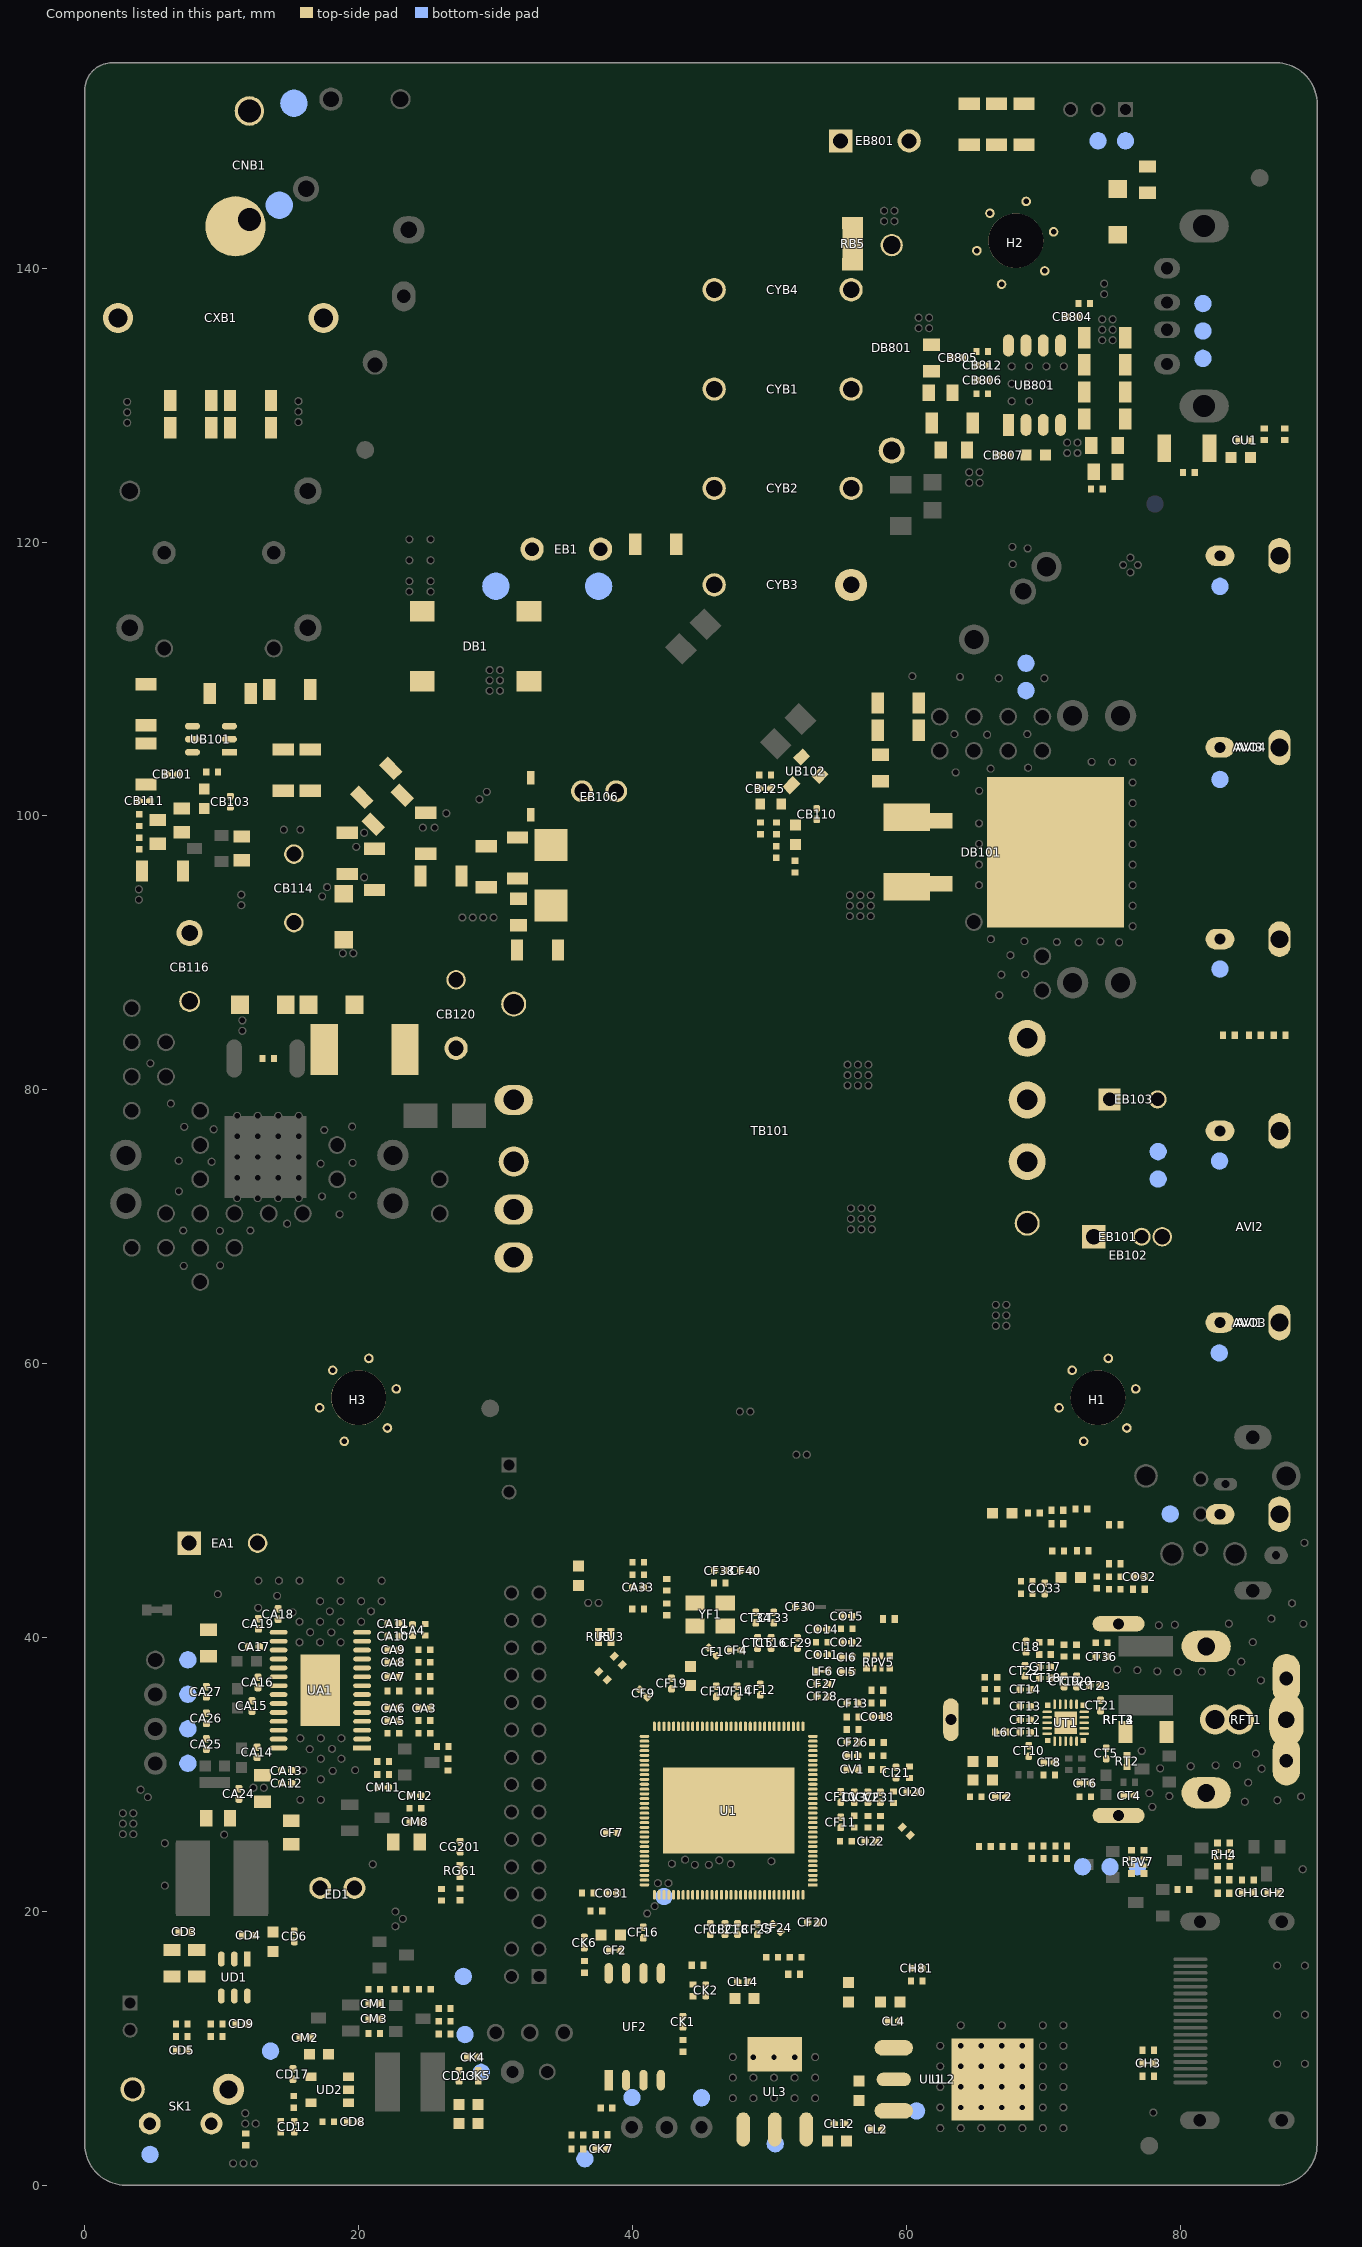
[diagram p0: the components of this part, seen from the top]
# Altium PCB MISC116569.PcbDoc (part 3 of 15)
Units mm, origin at the board's own origin, x right, y up, seen from the top; angles counter-clockwise.
Board outline 90 x 155 mm, 2 copper layers (TopLayer, BottomLayer), stack 1.571 mm thick; 527 components, 277 nets, 2450 pads, 649 vias.

## Components (designator, comment, footprint, x,y, rotation, side; value= is the part's Value field where it differs from the comment) (continued)
RA14 "1Kohm-0402-±1%-1/16W" R0402 24.862,40.57 r90 top
RA25 "10ohm-0402-±1%-1/16W" R0402 24.804,37.154 r0 top
RA31 "NC/1Kohm-0402-±1%-1/16W" R0402 75.217,44.44 r180 top
RA32 "NC/1Kohm-0402-±1%-1/16W" R0402 72.79,49.378 r180 top
RA33 "NC/Thick-film resistor,RES,1/16W,180ohm,±1%,0402,SMD" R0402 69.318,49.088 r0 top
RA34 "NC/Thick-film resistor,RES,1/16W,180ohm,±1%,0402,SMD" R0402 73.901,44.025 r90 top
RA35 "NC/47Kohm-0402-±1%-1/16W" R0402 40.419,45.494 r180 top
RA36 "NC/10Kohm-0402-±1%-1/16W" R0402 40.413,44.579 r0 top
RB1 "1M2ohm-1206-±5%-1/4W" R1206 12.103,130.341 r180 top
RB2 "1M2ohm-1206-±5%-1/4W" R1206 12.103,128.347 r180 top
RB3 "1M2ohm-1206-±5%-1/4W" R1206 7.73,128.351 r180 top
RB4 "1M2ohm-1206-±5%-1/4W" R1206 7.73,130.345 r180 top
RB5 "NC/Thick-film resistor,RES,1/4W,0ohm,±5%,1206,SMD" R1206SC 56.07,141.798 r90 top
RB101 "Thick-film resistor,RES,1/4W,330Kohm,±1%,1206,SMD" R1206 14.96,109.24 r180 top
RB102 "Thick-film resistor,RES,1/4W,330Kohm,±1%,1206,SMD" R1206 10.631,108.95 r180 top
RB103 "6K8ohm-0402-±1%-1/16W" R0402 3.975,99.695 r270 top
RB104 "47Kohm-0402-±1%-1/16W" R0402 9.296,103.2 r0 top
RB105 "510ohm-0402-±1%-1/16W" R0402 3.975,97.987 r270 top
RB106 "68ohm-0805-±5%-1/8W" R0805 11.455,97.638 r270 top
RB107 "20ohm-0805-±5%-1/8W" R0805 7.087,99.682 r270 top
RB109 "10Kohm-0402-±1%-1/16W" R0402 13.398,82.283 r180 top
RB114 "4R7ohm-1206-±1%-1/4W" R1206 33.06,90.208 r0 top
RB116 "NC/10ohm-1206-±5%-1/4W" R1206 31.598,96.926 r270 top
RB117 "Thick-film resistor,RES,1/4W,10ohm,±1%,1206,SMD" R1206 16.472,103.347 r90 top
RB118 "Thick-film resistor,RES,1/4W,10ohm,±1%,1206,SMD" R1206 14.488,103.347 r90 top
RB119 "Thick-film resistor,RES,1/4W,10ohm,±1%,1206,SMD" R1206 5.677,95.974 r0 top
RB121 "NC/Thick-film resistor,RES,1/8W,27Kohm,±1%,0805,SMD" R0805 5.334,98.842 r90 top
RB123 "47ohm-1206-±5%-1/4W" R1206 59.413,106.265 r0 top
RB124 "47ohm-1206-±5%-1/4W" R1206 59.413,108.246 r0 top
RB125 "Thick-film resistor,RES,1/4W,100Kohm,±1%,1206-Auto,SMD" R1206 19.168,97.262 r90 top
RB126 "Thick-film resistor,RES,1/4W,100Kohm,±1%,1206-Auto,SMD" R1206 21.285,102.413 r45 top
RB127 "Thick-film resistor,RES,1/4W,100Kohm,±1%,1206-Auto,SMD" R1206 21.161,96.094 r90 top
RB128 "Thick-film resistor,RES,1/4W,100Kohm,±1%,1206-Auto,SMD" R1206 22.123,100.457 r45 top
RB130 "Thick-film resistor,RES,1/4W,20ohm,±1%,1206,SMD" R1206 41.689,119.842 r0 top
RB131 "Thick-film resistor,RES,1/10W,2Kohm,±1%,0603,SMD" R0603 50.097,100.863 r0 top
RB132 "Thick-film resistor,RES,1/16W,1.2Kohm,±1%,0402,SMD" R0402 49.677,102.984 r180 top
RB133 "10Kohm-0402-±1%-1/16W" R0402 51.862,96.298 r270 top
RB134 "4K7ohm-0402-±1%-1/16W" R0402 50.503,97.365 r90 top
RB135 "18Kohm-0402-±1%-1/16W" R0402 50.516,99.092 r270 top
RB141 "NC/Thick-film resistor,RES,1/4W,2Mohm,±5%,1206,SMD" R1206 4.478,108.121 r90 top
RB142 "NC/Thick-film resistor,RES,1/4W,2Mohm,±5%,1206,SMD" R1206 4.478,103.791 r90 top
RB148 "Thick-film resistor,RES,2W,0.36ohm,±5%,2512,SMD" R2512-1 20.434,82.944 r180 top
RB158 "NC/Thick-film resistor,RES,1/16W,51ohm,±1%,0402,SMD" R0402 49.347,99.092 r270 top
RB161 "Thick-film resistor,RES,1/4W,510Kohm,±1%,1206,SMD" R1206 24.905,98.742 r270 top
RB162 "Thick-film resistor,RES,1/4W,510Kohm,±1%,1206,SMD" R1206 26.011,95.606 r0 top
RB163 "Thick-film resistor,RES,1/4W,510Kohm,±1%,1206,SMD" R1206 29.316,96.287 r90 top
RB801 "Thick-film resistor,RES,1/16W,100ohm,±1%,0402,SMD" R0402 73.915,123.888 r180 top
RB803 "10Kohm-0402-±1%-1/16W" R0402 65.54,130.835 r0 top
RB804 "NC/10Kohm-0402-±5%-1/16W" R0402 65.54,133.921 r180 top
RB805 "Thick-film resistor,RES,1/16W,100ohm,±1%,0402,SMD" R0402 72.987,137.427 r0 top
RB810 "Thick-film resistor,RES,1/4W,10ohm,±1%,1206,SMD" R1206 74.493,128.981 r0 top
RB812 "Thick-film resistor,RES,1/4W,10ohm,±1%,1206,SMD" R1206 63.354,128.702 r180 top
RB814 "Thick-film resistor,RES,1/8W,390Kohm,±1%,0805-Auto,SMD" R0805 62.505,130.899 r180 top
RB816 "Thick-film resistor,RES,1/8W,10ohm,±1%,0805,SMD" R0805 74.557,125.146 r180 top
RB818 "0R2ohm-1206-±1%-1/4W" R1206 74.493,134.928 r180 top
RB819 "0R1ohm-1206-±1%-1/4W" R1206 74.493,132.946 r180 top
RB820 "0R1ohm-1206-±1%-1/4W" R1206 74.493,130.963 r180 top
RB837 "1R6ohm-1206-±1%-1/4W" R1206 64.586,150.512 r90 top
RB838 "2R2ohm-1206-±1%-1/4W" R1206 66.589,150.512 r90 top
RB839 "2R2ohm-1206-±1%-1/4W" R1206 68.591,150.512 r270 top
RD1 "100Kohm-0402-±1%-1/16W" R0402 9.628,10.858 r0 top
RD3 "Thick-film resistor,RES,1/16W,60.4Kohm,±1%,0402,SMD" R0402 7.076,10.858 r180 top
RD5 "Thick-film resistor,RES,1/16W,10.5Kohm,±1%,0402,SMD" R0402 7.076,11.773 r0 top
RD6 "NC/?" R0402 9.628,11.773 r0 top
RD7 "Thick-film resistor,RES,1/16W,100Kohm,±1%,0402,SMD" R0402 17.782,4.638 r180 top
RD8 "Thick-film resistor,RES,1/16W,13Kohm,±1%,0402,SMD" R0402 15.261,6.083 r90 top
RD9 "Thick-film resistor,RES,1/16W,12Kohm,±1%,0402,SMD" R0402 14.308,4.27 r90 top
RF3 "NC/4K7ohm-0402-±5%-1/16W" R0402 38.101,5.641 r0 top
RF8 "4K7ohm-0402-±1%-1/16W" R0402 71.317,23.863 r0 top
RF9 "4K7ohm-0402-±1%-1/16W" R0402 50.198,16.652 r0 top
RF12 "68ohm-0402-±5%-1/16W" R0402 56.071,33.287 r180 top
RF13 "4K7ohm-0402-±1%-1/16W" R0402 27.414,21.237 r270 top
RF16 "68ohm-0402-±5%-1/16W" R0402 58.102,26.537 r270 top
RF25 "Thick-film resistor,RES,1/16W,1.3Kohm,±1%,0402,SMD" R0402 46.375,43.97 r180 top
RF29 "4K7ohm-0402-±1%-1/16W" R0402 37.364,20.03 r180 top
RF43 "4K7ohm-0402-±1%-1/16W" R0402 70.124,38.75 r0 top
RF44 "4K7ohm-0402-±1%-1/16W" R0402 70.124,39.652 r0 top
RFT1 "RF jack,RF JACK,H,IEC,T14.5,CH6.3,12.4×13.2×7.7mm,DIP,LHD-020 assembly,LHD" ANT-IEC14.5-H-4 88,34 r90 top locked
RFT2 "NC/RF shield can,RF SHLED,Single,H,IEC,T14.5,CH6.3,whole,14.5×25×9,DIP,122010461,VAST" T-14.5×25×9.0-IEC14.5 87.75,34 r90 top locked
RFT3 "NC/T-25×14.5×9-IEC14.5-LHD (3 pins)" T-25×14.5×9-IEC14.5-LHD-1 87.75,34 r90 top locked
RFT4 "NC/RF shield can,RF SHLED,Single,H,F,T14.5,CH6.3,whole,25.0×14.5×10.0mm,DIP,T-14.5×25×10-F14.5-LHD" T-14.5×25×10-F14.5 89.7,34 r90 top locked
RG61 "NC/" R0402SC#1 27.414,22.951 r90 top
RH3 "1Kohm-0402-±1%-1/16W" R0402 84.945,22.278 r180 top
RH4 "Resistor array,RES ARRAY,1/16W,4×10Kohm,±5%,0402,SMD" RA0402 83.172,24.144 r180 top
RH5 "33ohm-0402-±1%-1/16W" R0402 69.583,24.778 r180 top
RH6 "33ohm-0402-±1%-1/16W" R0402 69.583,23.863 r180 top
RH59 "1Kohm-0402-±1%-1/16W" R0402 80.234,21.605 r180 top
RH81 "22Kohm-0402-±1%-1/16W" R0402 67.456,24.74 r0 top
RH82 "33Kohm-0402-±1%-1/16W" R0402 65.742,24.74 r180 top
RH83 "100ohm-0402-±1%-1/16W" R0402 60.765,14.925 r0 top
RH88 "100ohm-0402-±1%-1/16W" R0402 71.305,24.778 r0 top
RH89 "100ohm-0402-±1%-1/16W" R0402 51.906,16.652 r180 top
RI3 "33ohm-0402-±1%-1/16W" R0402 57.912,31.369 r180 top
RI15 "Thick-film resistor,RES,1/16W,0ohm,±1%,0402,SMD" R0402 68.796,43.193 r180 top
RI16 "NC/Thick-film resistor,RES,1/16W,0ohm,±1%,0402,SMD" R0402 75.217,43.523 r180 top
RI18 "75ohm-0402-±1%-1/16W" R0402 57.921,32.334 r180 top
RK3 "1Kohm-0402-±1%-1/16W" R0402 44.42,14.226 r270 top
RK4 "4K7ohm-0402-±1%-1/16W" R0402 43.683,10.175 r90 top
RK10 "1Kohm-0402-±1%-1/16W" R0402 21.135,11.09 r180 top
RK12 "4K7ohm-0402-±1%-1/16W" R0402 35.981,3.673 r180 top
RK13 "33Kohm-0402-±1%-1/16W" R0402 26.278,11.979 r0 top
RK14 "510ohm-0402-±1%-1/16W" R0402 26.278,11.051 r0 top
RK15 "10Kohm-0402-±1%-1/16W" R0402 26.278,12.906 r0 top
RK18 "22ohm-0402-±1%-1/16W" R0402 35.981,2.657 r180 top
RK19 "1Kohm-0402-±1%-1/16W" R0402 36.482,15.941 r90 top
RM1 "10Kohm-0402-±1%-1/16W" R0402 40.406,42.078 r180 top
RM2 "4K7ohm-0402-±1%-1/16W" R0402 21.135,14.313 r180 top
RM3 "4K7ohm-0402-±1%-1/16W" R0402 24.842,14.313 r180 top
RM4 "Thick-film resistor,RES,1/16W,100Kohm,±1%,0402,SMD" R0402 23.055,14.313 r180 top
RM11 "4K7ohm-0402-±1%-1/16W" R0402 26.525,30.721 r90 top
RM12 "10Kohm-0402-±1%-1/16W" R0402 26.144,32.029 r0 top
RM13 "4K7ohm-0402-±1%-1/16W" R0402 21.782,29.989 r0 top
RM14 "47Kohm-0402-±1%-1/16W" R0402 21.782,30.932 r180 top
RM15 "NC/4K7ohm-0402-±5%-1/16W" R0402 24.15,27.533 r0 top
RO2 "NC/0ohm-0402-±5%-1/16W" R0402 68.79,44.107 r0 top
RO4 "NC/0ohm-0402-±5%-1/16W" R0402 71.077,46.319 r0 top
RO12 "NC/510ohm-0402-±1%-1/16W" R0402 53.818,39.652 r0 top
RO15 "NC/510ohm-0402-±1%-1/16W" R0402 55.646,40.642 r0 top
RO17 "NC/0ohm-0402-±5%-1/16W" R0402 57.868,35.204 r0 top
RO18 "NC/Thick-film resistor,RES,1/16W,75ohm,±1%,0402,SMD" R0402 56.071,34.194 r180 top
RO21 "NC/Thick-film resistor,RES,1/16W,150ohm,±1%,0402,SMD" R0402 36.736,21.339 r0 top
RO22 "NC/75ohm-0402-±1%-1/16W" R0402 26.056,21.209 r90 top
ROUT+ "DM0" TP 7.526,38.371 r180 bottom
ROUT- "DM0" TP 7.526,35.851 r180 bottom
RPV5 "Resistor array,RES ARRAY,1/16W,4×10Kohm,±5%,0402,SMD" RA0402 57.936,38.199 r90 top
RPV7 "Resistor array,RES ARRAY,1/16W,4×4.7Kohm,±5%,0402,SMD" RA0402 76.901,23.608 r0 top
RT1 "Ferrite bead,BEAD,120ohm,0402,800mA,SMD,TP,CBM100505U121T,FH" R0402 65.07,28.374 r0 top
RT2 "NC/" R0402SC#2 76.119,30.978 r270 top
RT5 "Thick-film resistor,RES,1/16W,51Kohm,±1%,0402,SMD" R0402 74.257,39.611 r0 top
RT10 "Thick-film resistor,RES,1/16W,100ohm,±1%,0402,SMD" R0402 65.724,36.676 r90 top
RT12 "NC/" R0402 66.175,35.368 r180 top
RT13 "Thick-film resistor,RES,1/16W,100ohm,±1%,0402,SMD" R0402 66.638,36.676 r90 top
RT14 "Thick-film resistor,RES,1/16W,100ohm,±1%,0402,SMD" R0402 71.521,39.048 r90 top
RT15 "Thick-film resistor,RES,1/16W,100ohm,±1%,0402,SMD" R0402 72.436,39.048 r90 top
RU3 "NC/0ohm-0402-PCB" R0402SC#1 38.431,40.046 r90 top
RU4 "Thick-film resistor,RES,1/16W,0ohm,±1%,0402,SMD" R0402 80.64,125.07 r180 top
RU5 "NC/0ohm-0402-PCB" R0402SC#1 37.518,40.046 r90 top
RV1 "Thick-film resistor,RES,1/16W,75ohm,±1%,0402,SMD" R0402 60.236,30.156 r90 top
RV2 "Thick-film resistor,RES,1/16W,33ohm,±1%,0402,SMD" R0402 57.859,30.366 r180 top
RV3 "Thick-film resistor,RES,1/16W,75ohm,±1%,0402,SMD" R0402 59.055,28.334 r90 top
RV4 "Thick-film resistor,RES,1/16W,33ohm,±1%,0402,SMD" R0402 57.188,26.537 r90 top
RV5 "Thick-film resistor,RES,1/16W,75ohm,±1%,0402,SMD" R0402 55.582,25.121 r0 top
RV10 "Thick-film resistor,RES,1/16W,33ohm,±1%,0402,SMD" R0402 56.195,26.558 r90 top
S/N1 "Barcode" BARCODE 53.154,56.375 r0 top
S/N2 "Barcode" BARCODE 52.946,44.901 r0 bottom
SFQ1 "NC/Conformal coating,25kg/Can,Peters" SFQ 6.985,82.474 r0 top
SFQ2 "NC/Conformal coating,25kg/Can,Peters" SFQ 20.013,108.255 r180 top
SFQ3 "NC/Conformal coating,25kg/Can,Peters" SFQ 52.362,92.113 r90 top
SFQ4 "NC/Conformal coating,25kg/Can,Peters" SFQ 74.79,120.046 r90 top
SK1 "Tact switch,Tact Switch,160±50gf,7.0×10.3×7.0mm,DIP,106520070,VAST" KEY-HD-6 6.996,2 r0 top locked
TB101 "变压器,Transformer,EQ2414,300uH,0.2×1P,26Ts,H14.5MAX,SYEQ2414Z-T012064B(BLACK),DIP,SQ" T/EQ2414*10 52.823,77.006 r0 top locked
TP-TDT "NC/" TP-TDT 33.773,116.776 r0 bottom
TP_12VA+ "NC/" TP 68.745,109.15 r180 bottom
TP_12VA- "NC/" TP 78.389,73.482 r180 bottom
TP_12VB+ "NC/" TP 68.745,111.15 r180 bottom
TP_12VB- "NC/" TP 78.389,75.482 r180 bottom
TP_L "NC/" TP-80 15.273,152.044 r180 bottom
TP_LED+ "NC/" TP 76.002,149.305 r180 bottom
TP_LED- "NC/" TP 74.002,149.305 r180 bottom
TP_N "NC/" TP-80 14.206,144.602 r180 bottom
U1 "TV main chip,IC Main Chip,TSUMV53RWET,32bit,Single-Core,QFN128,SMD,Mstar" QFN128/0.35-1 47.024,27.357 r180 top locked
UA1 "Audio amplifier,IC Audio AMP,Class D,2X8W@12V@8ohm,E-TSSOP-28L,SMD,AD52050B-26QG28NRR,ESMT" SOP28/0.65-7 17.204,36.154 r180 top locked
UART_RX "" TP 72.873,23.254 r180 bottom
UART_TX "" TP 74.873,23.254 r180 bottom
UB101 "PWM controller,IC PWM Controller,100KHZ,SOT23-6,SMD,LD5537B3GL,Leadtrend" SOT-26 9.207,105.6 r270 top
UB102 "Voltage regulator,IC Regulator,2.50V,0.4%,SOT-23,SMD,BR431M-A,Blue Rocket" SOT-23-RAK 52.3,102.913 r135 top
UB801 "PWM controller,IC PWM Controller,120KHz,SOP-8,SMD,OB33510CPA,ON-Bright" SO-8A 69.363,131.458 r90 top
UD1 "DC-DC converter,IC DC-DC,Syn,3A,18V,600KHz,SOT23-6,SMD,TMI3253T,TOLL" TSOT23-6 10.917,15.175 r270 top
UD2 "DC-DC converter,IC DCDC,Syn,1.2A,6.0V,1.5MHz,SOT23-5,SMD,TMI3408,TOLL" SOT-23-5 17.899,6.975 r90 top
UF2 "SPI FLASH chip,IC SPI FLASH,4MB,32Mb,SOIC8,SMD,W25Q32JVSSIQ,Winbond" SOIC8 40.165,11.571 r90 top locked
UL1 "LDO regulator,IC LDO,1A,3.3V,15V,SOT223,SMD,SCJT1117B-3.3V,CJKJ" SOT-223 61.83,7.728 r270 top
UL2 "NC/LC1117COTR33" TO-252 62.68,7.728 r270 top
UL3 "LDO regulator,IC LDO,1A,1.8V,12V,SOT-223,SMD,LC1117CLTR18,Leadchip" SOT-223 50.389,6.822 r0 top
UT1 "Silicon tuner chip,IC Si Tuner,QFN-24,SMD,ATBM253,AltoBeam" QFN24/0.4-1 71.632,33.772 r180 top locked
VCC_PANEL "TEST" TP 27.643,15.251 r90 bottom
VDDC_CORE "TEST" TP 42.304,21.082 r90 bottom
XXXXXX "PCB_TIME" PCB_TIME 49.974,59.804 r90 bottom
XXXXXXXXXXXXX "PCB_NAME" PCB_NAME 52.984,59.893 r90 top
Y_Pb_LOUT "DM0" TP 82.901,102.669 r90 bottom
Y_Pr_ROUT "DM0" TP 82.901,116.766 r90 bottom
Y_Y_AV_OUT "DM0" TP 82.901,88.814 r90 bottom
YF1 "Passive crystal,SPXO,24MHz,±10ppm,12pF,SMD3225,SMD,2.3.3.240001234,MDH" XTAL-S-3 45.669,41.683 r0 top locked
YPBPR_L/AV_L "DM0" TP 82.85,60.785 r90 bottom
YPBPR_R/AV_R "DM0" TP 82.875,74.793 r90 bottom
用于U1上 "NC/Glue,0.1g,silicone,ZJ" "Heat-Shrinkable Tube" 35.865,5.359 r90 top

## Footprints (in the part's own frame and the unit in brackets; to place one, negate y for a bottom-side part, rotate by r counter-clockwise, add the part's x,y. Pads: shape width x height; smd on the part's side, far side on the other; paste and mask are expansions set on the pad)
ANT-IEC14.5-H-4 [mm] "联宏达；13.2×12.4×7.7mm LHD-020 中心高度6.3mm 160323(18.03.09更新脚距）,向内扩宽丝印,0703_2018（18.08.29 更新短槽孔）"
  oval 2.5x3.8 on Top Overlay paste-4 mask-4: 0(-5.35,6.1) 0(5.35,6.1)
  round 2.4 on Top Overlay: 0(0,5.45)
  oval 4.1x2.7 on Top Overlay paste-4 mask-4: 0(0,0.25)
  round 2.2 hole 1.4: 1(0,5.45)
  oval 2.3x3.6 hole 1.3 slot 2.6 at 90 deg: 2(-5.35,6.1) 4(5.35,6.1)
  oval 3.9x2.5 hole 1.2 slot 2.6 at 0 deg: 3(0,0.25)
  KeepOutLayer pour cut-out: 0,3.95 -0.574,4.064 -1.061,4.389 -1.386,4.876 -1.5,5.45 -1.5,5.45 -1.386,6.024 -1.061,6.511 -0.574,6.836 0,6.95 0,6.95 0.574,6.836 1.061,6.511 1.386,6.024 1.5,5.45 1.5,5.45 1.386,4.876 1.061,4.389 0.574,4.064 0,3.95
  silkscreen extent -6.3,0 6.3,7.9, body extent -7.55,-35.2 7.55,7.7, height 13.76
ASSE4.0C-3 [mm] "定位孔(顶底层上锡)(17.12.09更新过孔位置）18.11.22 更新paste形状为扇形。"
  round 4 hole 4 unplated mask+0: 0(0,0)
  round 0.7 hole 0.4: 1(-2.85,-0.725) 2(-1.893,2.011) 3(0.75,2.875) 4(2.75,0.65) 5(2.105,-2.203) 6(-1.05,-3.175)
  KeepOutLayer pour cut-out: 0,-2.3 -0.88,-2.125 -1.626,-1.626 -2.125,-0.88 -2.3,0 -2.3,0 -2.125,0.88 -1.626,1.626 -0.88,2.125 0,2.3 0,2.3 0.88,2.125 1.626,1.626 2.125,0.88 2.3,0 2.3,0 2.125,-0.88 1.626,-1.626 0.88,-2.125 0,-2.3
AV2-H14-15 [mm] "宇球；RC086-F02L3BY-X; 中心高度：5.5mm;160307；170802加大接地脚焊盘（18.03.09更新孔径）"
  oval 2.8x2.5 on Top Overlay: 0(-7,2.75) 0(7,2.75)
  oval 1.7x2.7 on Top Overlay: 0(-7,7.1) 0(7,7.1)
  oval 1.5x2.108 / inner oval 1.5x2.5 / far side oval 1.5x2.5 hole 0.8 slot 1.8 at 90 deg: 1(-7,7.1) 3(7,7.1)
  oval 2.6x1.626 / inner oval 2.6x2.3 / far side oval 2.6x2.3 hole 1.3 slot 1.6 at 0 deg: 2(-7,2.75) 4(7,2.75)
  silkscreen extent -13.3,0 13.3,7.8, body extent -13.1,-8.9 13.1,8, height 10.7
AV3-H14-15 [mm] "宇球；RC075-F03L3BY-A; 中心高度：5.5mm;15.11.24;170401兼容物料，更新高度;170802加大接地脚焊盘（18.03.09更新孔距）"
  oval 2.8x2.5 on Top Overlay: 0(-14,2.75) 0(0,2.75) 0(14,2.75)
  oval 1.7x2.7 on Top Overlay: 0(-14,7.1) 0(0,7.1) 0(14,7.1)
  oval 1.5x2.108 / inner oval 1.5x2.5 / far side oval 1.5x2.5 hole 0.8 slot 1.8 at 90 deg: 1(-14,7.1) 3(0,7.1) 5(14,7.1)
  oval 2.6x1.626 / inner oval 2.6x2.3 / far side oval 2.6x2.3 hole 1.3 slot 1.6 at 0 deg: 2(-14,2.75) 4(0,2.75) 6(14,2.75)
  silkscreen extent -20.3,0 20.3,7.8, body extent -20.1,-9 20.1,7.9, height 10.7
B/YBS3010A [mm] "YJ,YBS3010A,18.04.17"
  rect 1.5x1.8 smd: 1(2.55,3.9) 2(2.55,-3.9) 3(-2.55,-3.9) 4(-2.55,3.9)
  silkscreen extent -3.35,-3.7 3.35,5.74, body extent -3.35,-3.7 3.35,3.7, height 1.5
BARCODE [mm] "(18.12.17 更新为白油）"
  round 0.3 on Mech2: 0(0,0)
  silkscreen extent -15,-4 15,4
C0402#1 [mm]
  rrect50% 0.45x0.5 smd mask+0.051: 1(-0.425,0) 2(0.425,0)
  rect 0.3x0.3 smd mask+0.051: 1(-0.25,0) 2(0.25,0)
  rect 0.6x0.6 on Top Solder: 2(0,0)
  TopLayer pour cut-out: -0.318,0.302 -0.318,-0.303 0.306,-0.303 0.306,0.302
  silkscreen extent -0.88,-0.4 0.88,0.4, body extent -0.5,-0.25 0.5,0.25, height 0.5
C0402#2 [mm]
  rect 0.45x0.5 smd mask+0.076: 1(-0.425,0) 2(0.425,0)
  silkscreen extent -0.88,-0.4 0.88,0.4, body extent -0.5,-0.25 0.5,0.25, height 0.5
C0603 [mm] "片式电容"
  rect 0.8x0.8 smd mask+0.076: 1(-0.706,0) 2(0.706,0)
  silkscreen extent -1.39,-0.62 1.39,0.62, body extent -0.8,-0.4 0.8,0.4, height 0.8
C0805 [mm] "片式电容"
  rect 0.9x1.25 smd mask+0.076: 1(-0.966,0) 2(0.966,0)
  silkscreen extent -1.73,-0.84 1.73,0.84, body extent -1,-0.62 1,0.63, height 1.25
C1206 [mm] "片式电容"
  rect 1x1.6 smd mask+0.076: 1(-1.5,0) 2(1.5,0)
  silkscreen extent -2.39,-1.02 2.39,1.02, body extent -1.6,-0.8 1.6,0.8, height 1.3
CAP6.5*5-V-5-1 [mm] "TDK，CC45SL3DD680JYSNA，外K型引脚，AI，0713_2018"
  round 2.1 on Top Overlay: 0(-2.5,0) 0(2.5,0)
  round 1.9 hole 1.2 mask+0.051: 1(-2.5,0)
  round 1.524 / inner round 1.9 / far side oval 1.9x1.651 hole 1.2 mask+0.051: 2(2.5,0)
  BottomLayer lines w0.6: 2.19,-0.39 4.056,-1.556 ; -2.89,-0.31 -4.056,1.556 ; 2.5,0 4.056,-1.556 ; -2.5,0 -4.056,1.556 ; 2.89,0.31 4.056,-1.556 ; -2.19,0.39 -4.056,1.556
  silkscreen extent -5.5,-2.5 5.5,2.5
CAP8*2.5-V-5 [mm] "C242G472J20A201(编带/法拉)"
  round 1.422 / inner round 1.8 / far side round 1.8 hole 1.1: 1(-2.5,0) 2(2.5,0)
  round 2 on Top Overlay: 1(-2.5,0) 1(2.5,0)
  BottomLayer lines w0.6: 2.15,-0.456 4.056,-1.556 ; -2.956,-0.35 -4.056,1.556 ; 2.5,0 4.056,-1.556 ; -2.5,0 -4.056,1.556 ; 2.956,0.35 4.056,-1.556 ; -2.15,0.456 -4.056,1.556
  silkscreen extent -4,-1.25 4,1.25
CAP10*4.5-V-5 [mm] "YU102472M090DAND5H，陶瓷电容，17.12.22"
  round 1.7 hole 1.1: 1(-2.5,0)
  round 1.422 / inner round 1.7 / far side round 1.7 hole 1.1: 2(2.5,0)
  round 1.9 on Top Overlay: 41(2.5,0) 42(-2.5,0)
  BottomLayer lines w0.6: -2.19,0.39 -2.238,0.42 -2.33,0.477 -2.5,0.584 -2.579,0.633 -2.769,0.751 -3.783,1.385 -4.056,1.556 ; 2.89,0.31 2.92,0.262 ; -2.5,0 -2.579,0.079 -2.769,0.269 -4.056,1.556 ; 2.5,0 3.275,-0.775 4.056,-1.556 ; -2.89,-0.31 -2.92,-0.262 -2.977,-0.17 -3.035,-0.078 -3.084,0 -4.056,1.556 ; 2.19,-0.39 2.238,-0.42 ; 2.92,0.262 2.92,0.262 ; 2.92,0.262 3.084,0 3.275,-0.306 4.056,-1.556 ; 2.238,-0.42 2.238,-0.42 ; 2.238,-0.42 2.438,-0.545 2.5,-0.584 3.275,-1.068 4.056,-1.556
  silkscreen extent -5.55,-2.25 5.55,2.25
CAP13*5-V-10-1#1 [mm] "Walsin;YU1AH471M060DAMD0H;160718（18.03.15  更新孔径）"
  round 1.7 hole 1.2: 1(-5,0) 2(5,0)
  oval 2.55x1.9 on Top Overlay: 61(-5,0) 61(5,0)
  silkscreen extent -5.71,-3 5.81,3
CAP13*5-V-10-1#2 [mm] "Walsin;YU1AH471M060DAMD0H;160718（18.03.15  更新孔径）"
  round 1.7 hole 1.2: 1(-5,0)
  round 2.35 hole 1.2: 2(5,0)
  oval 2.55x1.9 on Top Overlay: 61(-5,0) 61(5,0)
  silkscreen extent -5.71,-3 5.81,3
CAP18*8.5-V-15 [mm] "PX334K3ID49H200D9R(凯励)(18.01.12更新孔径）(18.07.18 更新丝印框，加了公差）(09/29/2019添加白油块)"
  round 2.2 hole 1.4: 1(-7.5,0) 2(7.5,0)
  round 2.4 on Top Overlay: 77(7.5,0) 78(-7.5,0)
  silkscreen extent -9.28,-4.45 9.28,4.45, body extent -9.25,-4.45 9.25,4.45, height 14.5
CAUTION [mm]
  silkscreen extent -10.17,-3.72 12.33,4.08
COLD [mm]
CON2-H7.92 [mm] "因物料底部露金属，20170630增加1.8mm安规禁布"
  round 2.159 / inner round 3 / far side round 4.4 hole 1.7: 1(0,3.96)
  round 4.4 hole 1.7 copper offset -1.016,-0.508: 3(0,-3.96)
  round 3.2 on Top Overlay: 109(0,3.96) 110(0,-3.96)
  silkscreen extent -12,-5.94 3.03,7.09, body extent -11.46,-6.04 0.56,5.86, height 8.49
"Conformal Coating" [mm] "三防漆虚线框"
  round 0.3 on Mech2: 0(0,0)
CQC [mm]
D2-H-15 [mm] "GOOD-ARK;HER201G~HER208G;14-04-18"
  round 2.1 on Top Overlay: 15(-7.5,0) 16(7.5,0)
  round 1.9 hole 1.3: A(-7.5,0)
  round 1.626 hole 1.3: K(7.5,0)
  BottomLayer lines w0.6: -7.404,0.643 -5.3,0 ; 7.404,0.643 7.312,0.615 6.661,0.416 6.544,0.38 5.3,0 ; -7.5,0 -5.3,0 ; 7.5,0 6.661,0 5.3,0 ; -7.404,-0.643 -5.3,0 ; 7.404,-0.643 7.312,-0.615 6.985,-0.515 6.544,-0.38 5.3,0
  silkscreen extent -7.5,-1.8 7.5,1.8, body extent -7.92,-1.78 7.92,1.81, height 3.6
D2PAK3 [mm] "伟达电子；SFS1006G;增加TO-252兼容；160309"
  oval 2.794x1.143 smd: 1(5.541,-2.2) 3(5.542,2.4)
  rect 2.794x1.143 smd: 1(5.544,-2.2) 3(5.544,2.4)
  rect 3.4x2 smd paste-5 mask-5: 1(7.494,-2.44) 3(7.494,2.64)
  rect 10x11 smd paste-11 mask-11: 2(-3.356,0.1)
  rect 6x6 smd paste-10 mask-11: 2(-2.158,0.1)
  TopLayer pour cut-out: 3.373,2.4 6.497,2.4 6.497,-2.245 6.438,-2.54 6.271,-2.791 6.02,-2.958 5.725,-3.017 5.725,-3.017 5.725,-2.199 4.141,-2.199 4.141,-3.024 3.847,-2.966 3.598,-2.799 3.432,-2.55 3.373,-2.256 3.373,-2.256
  silkscreen extent -9.13,-5.69 4.84,5.89, body extent -6.91,-5.15 8.79,5.35, height 4.7
DIODE-S0402 [mm] "DVD上使用的ESD"
  rect 0.45x0.55 smd mask+0.051: A(-0.425,0) K(0.425,0)
  silkscreen extent -0.8,-0.43 0.91,0.43, body extent -0.5,-0.25 0.5,0.25, height 0.5
DIODE-S-1 [mm] "SK34(18.09.07 去除0805电阻兼容）"
  rect 2.33x2.4 smd: A(-2.21,0) K(2.21,0)
  silkscreen extent -3.8,-1.4 4.04,1.4, body extent -2.63,-1.13 2.37,1.13, height 2
DIODE-S-12 [mm] "Formosa MS ;BAV19WS THRU BAV21WS/PMEG2010BEA(高度为1.1mm)"
  rect 1x0.55 smd: A(1.35,0) K(-1.35,0)
  silkscreen extent -0.9,-0.67 0.9,0.68, body extent -1.35,-0.63 1.35,0.63, height 1
DIODE-S-14 [mm] "ROHM;FSL14"
  rect 1.3x1.35 smd: A(1.675,0) K(-1.675,0)
  silkscreen extent -1.55,-1 1.55,1, body extent -1.95,-1 1.95,1, height 1.08
DOLBY_AS2 [mm] "杜比认证预留框，两行印刷，规格35.0*5.4mm  19.05.15"
Double-D-SILK [mm] "Dolby Double-D Silkscreen"
  silkscreen extent -2.2,-1.52 2.2,1.52
EC(5*11)-V-2.5 [mm] "机插2.5间距"
  round 1.8 on Top Overlay: 0(-1.25,0) 0(1.25,0)
  round 0.5 on Keep-Out: 0(0,-0.787)
  round 1.6 hole 1.1: 1(-1.25,0) 2(1.25,0)
  BottomLayer lines w0.6: -1.64,-0.31 -2.806,1.556 ; -1.25,0 -2.806,1.556 ; -0.94,0.39 -2.806,1.556 ; 0.94,-0.39 0.988,-0.42 1.25,-0.584 2.151,-1.147 2.245,-1.206 2.789,-1.545 2.806,-1.556 ; 1.25,0 2.245,-0.995 2.789,-1.539 2.806,-1.556 ; 1.64,0.31 1.67,0.262 2.397,-0.901 2.708,-1.399 2.806,-1.556
  silkscreen extent -2.75,-2.75 3,2.75, body extent -2.48,-2.52 2.5,2.47, height 12.5
EC(6.3*11)-V-2.5 [mm] "机插2.5间距"
  round 0.5 on Keep-Out: 0(0,-0.889)
  round 1.6 hole 1.1: 1(-1.25,0) 2(1.25,0)
  round 1.8 on Top Overlay: 5(1.25,0) 6(-1.25,0)
  BottomLayer lines w0.6: -1.665,-0.275 -2.664,1.685 ; -1.25,0 -1.275,0.03 -2.664,1.685 ; -0.907,0.361 -2.664,1.685 ; 0.907,-0.361 2.664,-1.685 ; 1.25,0 2.664,-1.685 ; 1.665,0.275 2.664,-1.685
  silkscreen extent -3.17,-3.17 3.51,3.17, body extent -3,-3 2.98,2.99, height 12.5
EC(8*11)-V-3.5 [mm]
  rect 1.6x1.6 hole 1: 1(-1.75,0)
  rect 1.8x1.8 on Top Overlay: 1(-1.75,0)
  round 1.8 on Top Overlay: 1(1.75,0)
  round 1.321 / inner round 1.6 / far side round 1.6 hole 1: 2(1.75,0)
  silkscreen extent -4.25,-4.25 4.45,4.25, body extent -3.98,-3.98 4.01,4.01, height 12.51
EC(10*12)-V-5 [mm] "机插5间距"
  rect 1.9x1.9 on Top Overlay: 0(-2.5,0)
  round 0.5 on Keep-Out: 0(-0.75,0)
  round 1.9 on Top Overlay: 0(2.5,0)
  rect 1.7x1.7 hole 1.1: 1(-2.5,0)
  round 1.422 / inner round 1.7 / far side round 1.7 hole 1.1: 2(2.5,0)
  BottomLayer lines w0.6: -2.89,-0.31 -2.92,-0.262 -3.084,0 -4.056,1.556 ; -2.5,0 -4.056,1.556 ; -2.19,0.39 -2.238,0.42 -4.056,1.556 ; 2.19,-0.39 4.056,-1.556 ; 2.5,0 4.056,-1.556 ; 2.89,0.31 4.056,-1.556
  silkscreen extent -5.25,-5.25 5.57,5.25, body extent -4.98,-4.99 5.01,4.99, height 12.01
EC(10*12.5)-V-5#1 [mm] "机插5间距"
  round 0.5 on Keep-Out: 0(0.572,-2.667)
  rect 1.7x1.7 hole 1.1: 1(-2.5,0)
  rect 1.9x1.9 on Top Overlay: 1(-2.5,0)
  round 1.9 on Top Overlay: 1(2.5,0)
  round 1.422 / inner round 1.7 / far side round 1.7 hole 1.1: 2(2.5,0)
  BottomLayer lines w0.6: -2.89,-0.31 -2.92,-0.262 -3.112,0.045 -4.056,1.556 ; -2.5,0 -2.579,0.079 -2.828,0.328 -4.056,1.556 ; -2.19,0.39 -2.238,0.42 -2.422,0.535 -4.056,1.556 ; 2.19,-0.39 4.056,-1.556 ; 2.5,0 4.056,-1.556 ; 2.89,0.31 4.056,-1.556
  silkscreen extent -5.2,-5.21 5.57,5.21, body extent -4.98,-4.99 5.01,4.99, height 14.01
EC(10*12.5)-V-5#2 [mm] "机插5间距"
  round 0.5 on Keep-Out: 0(-0.75,0)
  rect 1.7x1.7 hole 1.1: 1(-2.5,0)
  rect 1.9x1.9 on Top Overlay: 1(-2.5,0)
  round 1.9 on Top Overlay: 1(2.5,0)
  round 1.7 hole 1.1: 2(2.5,0)
  BottomLayer lines w0.6: -2.89,-0.31 -2.92,-0.262 -4.056,1.556 ; -2.5,0 -4.056,1.556 ; -2.19,0.39 -2.195,0.393 -2.238,0.42 -2.5,0.584 -4.056,1.556 ; 2.19,-0.39 2.238,-0.42 2.5,-0.584 4.056,-1.556 ; 2.5,0 4.056,-1.556 ; 2.89,0.31 2.92,0.262 4.056,-1.556
  silkscreen extent -5.2,-5.21 5.57,5.21, body extent -4.98,-4.99 5.01,4.99, height 14.01
EC(13*30)-H-5 [mm]
  round 1.7 hole 1: 1(2.5,0) 2(-2.5,0)
  round 1.9 on Top Overlay: 53(-2.5,0)
  rect 1.9x1.9 on Top Overlay: 54(2.5,0)
  silkscreen extent -6.78,-35 6.78,0.51, body extent -6.34,-34.59 6.28,0.3, height 12.52
EVA(7*7*3) [mm] "7*7*3"
  silkscreen extent -4.5,-4.5 4.5,4.5
Fixed [mm] "麦拉片塑胶固定柱(4.50×6.49mm-尼龙-白色)"
  round 2.5 on Keep-Out: 0(0,0)
  silkscreen extent -1.9,-1.9 1.9,1.9
FUSE1.1A-S [mm] "保险丝：FSMD005-1206(FUZETEC)（兼容1206F8.00A063V 高度0.8mm），18.03.07）"
  rect 1x2 smd: 1(-1.65,0) 2(1.65,0)
  silkscreen extent -2.4,-1.2 2.4,1.2, body extent -1.75,-0.9 1.75,0.9, height 1